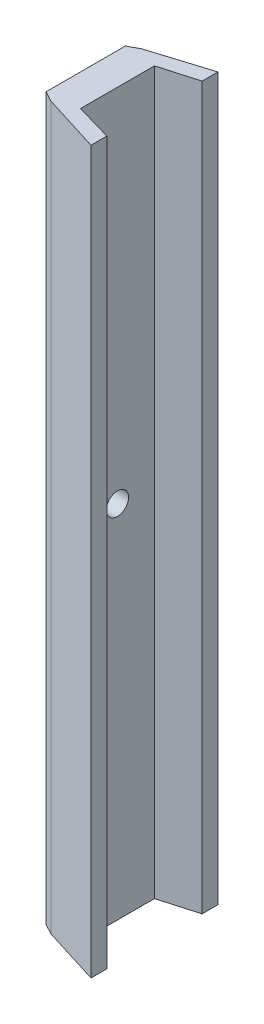
from build123d import *

# Parameters (mm, degrees)
BOSS_EXTRUDE1_DEPTH = 341
SKETCH2_R           = 10.5
CUT_EXTRUDE1_DEPTH  = 95


with BuildPart() as part:
    # Sketch1 → Boss-Extrude1 (new, symmetric)
    with BuildSketch(Plane(origin=(0, 0, 0), x_dir=(1, 0, 0), z_dir=(0, 1, 0))):
        Polygon((0, -37.5), (0, 37.5), (10, 42.881796684), (65, 60), (65, 45), (30, 35), (30, -35), (65, -45), (65, -60), (10, -42.881796684), align=None)
    extrude(amount=BOSS_EXTRUDE1_DEPTH, both=True)

    # Sketch2 → Cut-Extrude1 (cut)
    with BuildSketch(Plane.ZY):
        Circle(SKETCH2_R)
    extrude(amount=-CUT_EXTRUDE1_DEPTH, mode=Mode.SUBTRACT)


solid = part.part
